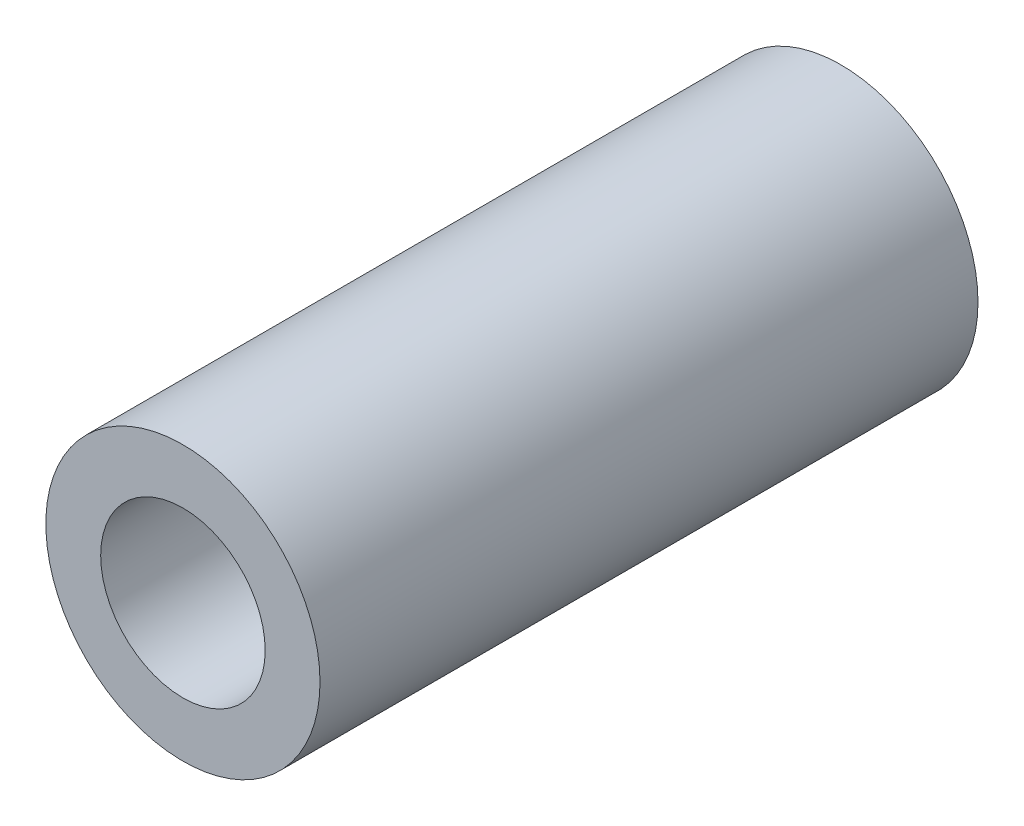
from build123d import *

# Parameters (mm, degrees)
SKETCH1_R           = 10
SKETCH1_R_2         = 6
BOSS_EXTRUDE1_DEPTH = 48


with BuildPart() as part:
    # Sketch1 → Boss-Extrude1 (new body)
    with BuildSketch(Plane.XY):
        Circle(SKETCH1_R)
        Circle(SKETCH1_R_2, mode=Mode.SUBTRACT)
    extrude(amount=BOSS_EXTRUDE1_DEPTH)


solid = part.part
